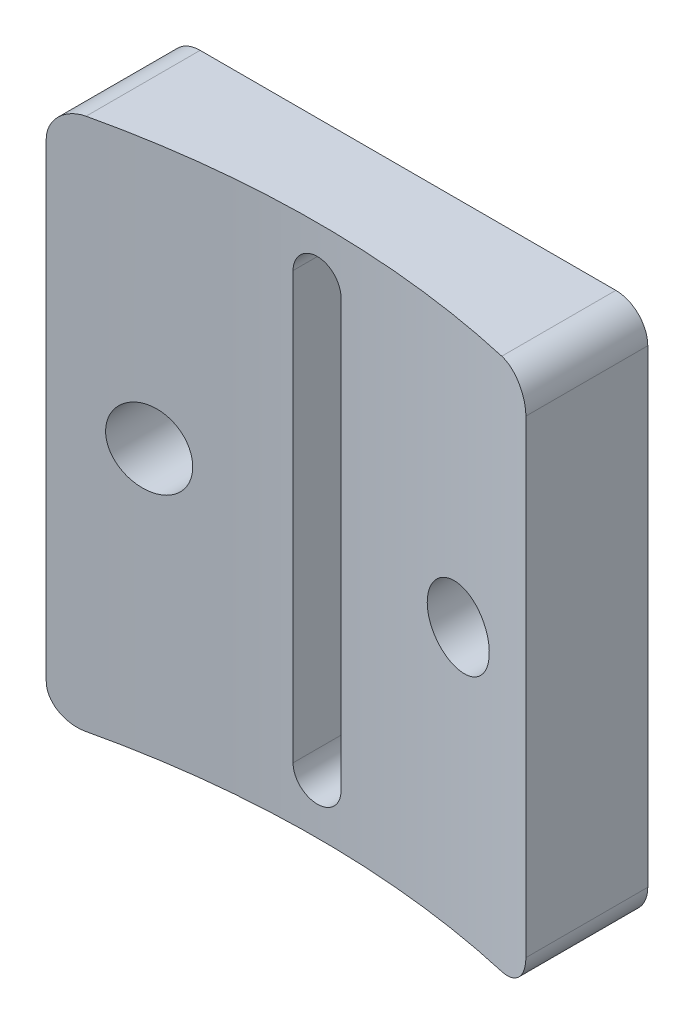
from build123d import *

# Parameters (mm, degrees)
BOSS_EXTRUDE1_DEPTH   = 50
M8X1_0_TAPPED_HOLE1_D = 7
CUT_EXTRUDE1_DEPTH    = 57.010506805
CUT_EXTRUDE2_DEPTH    = 4
FILLET1_R             = 3


with BuildPart() as part:
    # Sketch1 → Boss-Extrude1 (new body)
    with BuildSketch(Plane(origin=(0, 0, 0), x_dir=(1, 0, 0), z_dir=(0, 1, 0))):
        with BuildLine():
            Line((-22.5, 84.557672626), (-22.5, 96))
            Line((-22.5, 96), (22.5, 96))
            Line((22.5, 96), (22.5, 84.557672626))
            ThreePointArc((22.5, 84.557672626), (0, 87.5), (-22.5, 84.557672626))
        make_face()
    extrude(amount=BOSS_EXTRUDE1_DEPTH)

    # M8x1.0 Tapped Hole1 (through all)
    with Locations(Plane(origin=(0, 0, -96), x_dir=(-1, 0, 0), z_dir=(0, 0, -1))):
        with Locations((-14.5, 25), (14.5, 25)):
            Hole(M8X1_0_TAPPED_HOLE1_D / 2)

    # Sketch4 → Cut-Extrude1 (cut, through all)
    with BuildSketch(Plane(origin=(0, 0, -96), x_dir=(-1, 0, 0), z_dir=(0, 0, -1))):
        with BuildLine():
            Line((2.25, 45), (2.25, 5))
            ThreePointArc((2.25, 5), (0, 2.75), (-2.25, 5))
            Line((-2.25, 5), (-2.25, 45))
            ThreePointArc((-2.25, 45), (0, 47.25), (2.25, 45))
        make_face()
    extrude(amount=-CUT_EXTRUDE1_DEPTH, mode=Mode.SUBTRACT)

    # Sketch5 → Cut-Extrude2 (cut)
    with BuildSketch(Plane(origin=(0, 0, -96), x_dir=(-1, 0, 0), z_dir=(0, 0, -1))):
        with BuildLine():
            Line((4, 45), (4, 5))
            ThreePointArc((4, 5), (0, 1), (-4, 5))
            Line((-4, 5), (-4, 45))
            ThreePointArc((-4, 45), (0, 49), (4, 45))
        make_face()
    extrude(amount=-CUT_EXTRUDE2_DEPTH, mode=Mode.SUBTRACT)

    # Fillet1
    fillet1_edges = [part.edges().sort_by_distance(p)[0] for p in [
        (22.5, 50, -90.278836313),
        (22.5, 0, -90.278836313),
        (-22.5, 0, -90.278836313),
        (-22.5, 50, -90.278836313),
    ]]
    fillet(fillet1_edges, radius=FILLET1_R)


solid = part.part
